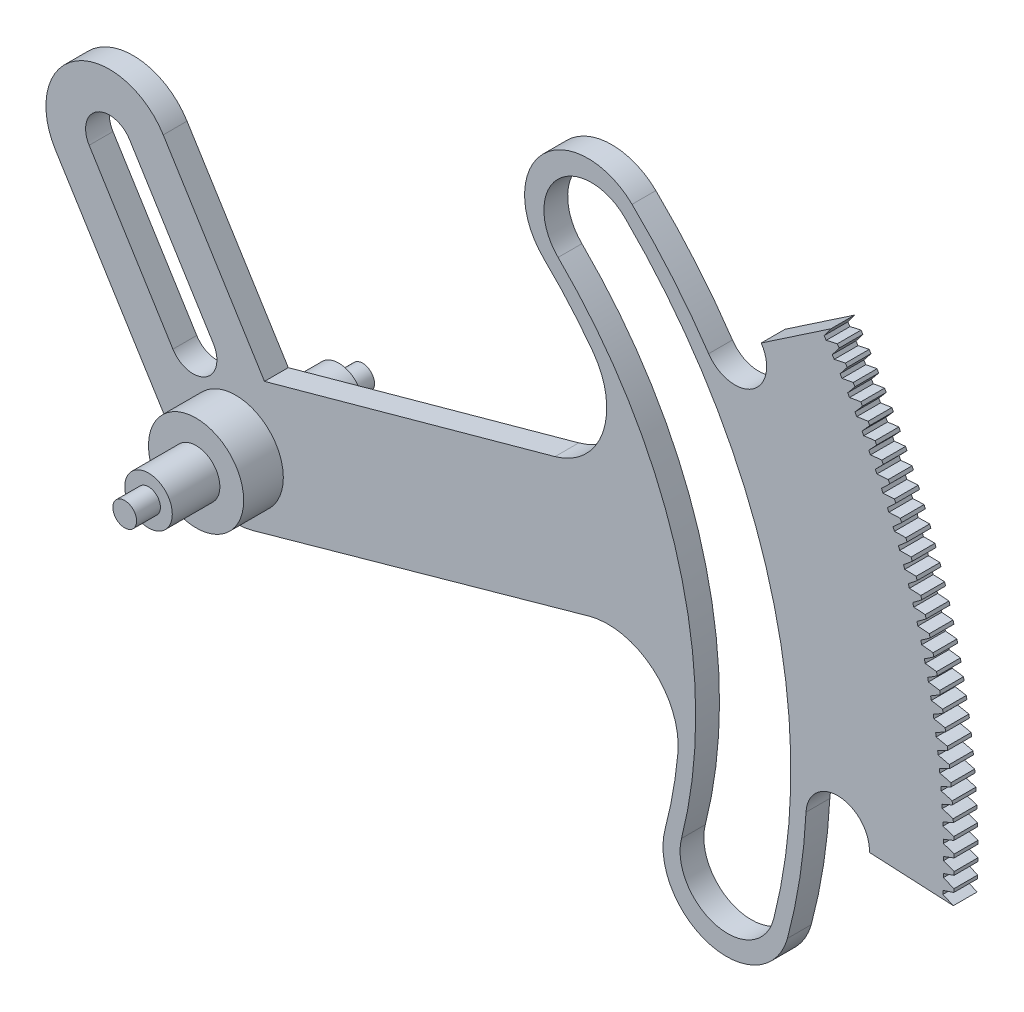
from build123d import *

# Parameters (mm, degrees)
BOSS_EXTRUDE_2_DEPTH = 1.5
BOSS_EXTRUDE_3_DEPTH = 1.5
SKETCH_12_R          = 3
BOSS_EXTRUDE_4_DEPTH = 2.5
SKETCH_13_R          = 1.5
BOSS_EXTRUDE_5_DEPTH = 3
SKETCH_14_R          = 0.75
BOSS_EXTRUDE_6_DEPTH = 1.5
BOSS_EXTRUDE_START   = 5
SKETCH_15_R          = 1.5
BOSS_EXTRUDE_7_DEPTH = 5
BOSS_EXTRUDE_START_2 = 1.5
SKETCH_16_R          = 0.75
BOSS_EXTRUDE_8_DEPTH = 1.5


with BuildPart() as part:
    # Sketch 6 → Boss-Extrude 2 (new body)
    with BuildSketch(Plane.XY):
        with BuildLine():
            Line((37.519779375, 25.38417136), (33.130048014, 22.414279348))
            ThreePointArc((33.130048014, 22.414279348), (32.59425958, 19.63706298), (29.817043212, 20.172851413))
            ThreePointArc((29.817043212, 20.172851413), (34.671419838, 9.689821796), (35.955419193, -1.791041762))
            ThreePointArc((35.955419193, -1.791041762), (38.052444802, 0.106979206), (39.95046577, -1.990046403))
            Line((39.95046577, -1.990046403), (45.243902486, -2.253727551))
            ThreePointArc((45.243902486, -2.253727551), (44.913502165, -2.110667794), (44.580306552, -1.974245108))
            ThreePointArc((44.580306552, -1.974245108), (44.58532509, -1.857461343), (44.590037698, -1.740664833))
            ThreePointArc((44.590037698, -1.740664833), (44.933425979, -1.632429188), (45.274580707, -1.517346967))
            ThreePointArc((45.274580707, -1.517346967), (45.278003129, -1.411535572), (45.281178259, -1.305716468))
            ThreePointArc((45.281178259, -1.305716468), (44.947854383, -1.169607468), (44.611874824, -1.040192624))
            ThreePointArc((44.611874824, -1.040192624), (44.614446527, -0.923329372), (44.6167121, -0.806459783))
            ThreePointArc((44.6167121, -0.806459783), (44.957758354, -0.691056496), (45.29642816, -0.568854908))
            ThreePointArc((45.29642816, -0.568854908), (45.297633885, -0.462995046), (45.298592211, -0.357132655))
            ThreePointArc((45.298592211, -0.357132655), (44.962490986, -0.228034115), (44.623874853, -0.105683879))
            ThreePointArc((44.623874853, -0.105683879), (44.623998593, 0.011207602), (44.623816137, 0.128099005))
            ThreePointArc((44.623816137, 0.128099005), (44.96237077, 0.250619317), (45.298407104, 0.379886669))
            ThreePointArc((45.298407104, 0.379886669), (45.297395602, 0.485748565), (45.296136703, 0.591607808))
            ThreePointArc((45.296136703, 0.591607808), (44.957405555, 0.713639262), (44.616301376, 0.828871224))
            ThreePointArc((44.616301376, 0.828871224), (44.613977098, 0.945739659), (44.611346694, 1.062601605))
            ThreePointArc((44.611346694, 1.062601605), (44.947261204, 1.1921852), (45.280516668, 1.328461615))
            ThreePointArc((45.280516668, 1.328461615), (45.277288384, 1.434279111), (45.273812812, 1.540088773))
            ThreePointArc((45.273812812, 1.540088773), (44.93260032, 1.654999613), (44.589157715, 1.763062756))
            ThreePointArc((44.589157715, 1.763062756), (44.584386438, 1.879856884), (44.579309239, 1.996638113))
            ThreePointArc((44.579309239, 1.996638113), (44.912436284, 2.133228151), (45.242764702, 2.276453854))
            ThreePointArc((45.242764702, 2.276453854), (45.237321051, 2.382180534), (45.231630331, 2.487894204))
            ThreePointArc((45.231630331, 2.487894204), (44.888086161, 2.595634028), (44.542455774, 2.696480953))
            ThreePointArc((44.542455774, 2.696480953), (44.535239593, 2.813149544), (44.527717825, 2.929798833))
            ThreePointArc((44.527717825, 2.929798833), (44.857911284, 3.0733354), (45.185167762, 3.223447568))
            ThreePointArc((45.185167762, 3.223447568), (45.177511134, 3.329037057), (45.169607762, 3.434608365))
            ThreePointArc((45.169607762, 3.434608365), (44.823882604, 3.535129912), (44.476216042, 3.628716381))
            ThreePointArc((44.476216042, 3.628716381), (44.46655812, 3.745208261), (44.456595084, 3.861674442))
            ThreePointArc((44.456595084, 3.861674442), (44.783710122, 4.01209458), (45.107751116, 4.169027369))
            ThreePointArc((45.107751116, 4.169027369), (45.097884867, 4.274433352), (45.08777231, 4.37981599))
            ThreePointArc((45.08777231, 4.37981599), (44.740017811, 4.47307517), (44.39046757, 4.559360135))
            ThreePointArc((44.39046757, 4.559360135), (44.378372145, 4.675624206), (44.36597221, 4.791856194))
            ThreePointArc((44.36597221, 4.791856194), (44.689865345, 4.949093922), (45.010548719, 5.112778496))
            ThreePointArc((45.010548719, 5.112778496), (44.998477178, 5.217954739), (44.986159871, 5.323102483))
            ThreePointArc((44.986159871, 5.323102483), (44.636528568, 5.40905839), (44.285247973, 5.488004003))
            ThreePointArc((44.285247973, 5.488004003), (44.270720349, 5.603989267), (44.255888955, 5.71993608))
            ThreePointArc((44.255888955, 5.71993608), (44.576418116, 5.883922429), (44.893603208, 6.05428699))
            ThreePointArc((44.893603208, 6.05428699), (44.879331669, 6.159187358), (44.864815015, 6.264054088))
            ThreePointArc((44.864815015, 6.264054088), (44.513460267, 6.342669017), (44.160603402, 6.414240651))
            ThreePointArc((44.160603402, 6.414240651), (44.143649953, 6.529896234), (44.126393604, 6.645507012))
            ThreePointArc((44.126393604, 6.645507012), (44.443418197, 6.816170053), (44.756965879, 6.993139873))
            ThreePointArc((44.756965879, 6.993139873), (44.740500602, 7.097718355), (44.723790969, 7.202258071))
            ThreePointArc((44.723790969, 7.202258071), (44.370866892, 7.27349754), (44.016588531, 7.3376638))
            ThreePointArc((44.016588531, 7.3376638), (43.997216692, 7.452938973), (43.977542959, 7.568163005))
            ThreePointArc((43.977542959, 7.568163005), (44.290923926, 7.745427879), (44.600696665, 7.928925334))
            ThreePointArc((44.600696665, 7.928925334), (44.582044873, 8.033136057), (44.56314959, 8.137302906))
            ThreePointArc((44.56314959, 8.137302906), (44.208810988, 8.201135667), (43.85326653, 8.257868408))
            ThreePointArc((43.85326653, 8.257868408), (43.831484798, 8.372712606), (43.80940231, 8.487499352))
            ThreePointArc((43.80940231, 8.487499352), (44.119002192, 8.671288304), (44.424864112, 8.861232906))
            ThreePointArc((44.424864112, 8.861232906), (44.404033986, 8.965030161), (44.382961341, 9.068778451))
            ThreePointArc((44.382961341, 9.068778451), (44.027363639, 9.125176505), (43.670709036, 9.174450842))
            ThreePointArc((43.670709036, 9.174450842), (43.646526966, 9.28881369), (43.622045409, 9.403112801))
            ThreePointArc((43.622045409, 9.403112801), (43.927728405, 9.593345216), (44.229545345, 9.789653649))
            ThreePointArc((44.229545345, 9.789653649), (44.206546021, 9.892991906), (44.183305258, 9.996276131))
            ThreePointArc((44.183305258, 9.996276131), (43.826604433, 10.045214739), (43.468996126, 10.087009059))
            ThreePointArc((43.468996126, 10.087009059), (43.442424325, 10.200840394), (43.415554437, 10.314601734))
            ThreePointArc((43.415554437, 10.314601734), (43.717186465, 10.51119417), (44.014826038, 10.713780326))
            ThreePointArc((44.014826038, 10.713780326), (43.989667605, 10.816614257), (43.964268917, 10.919389113))
            ThreePointArc((43.964268917, 10.919389113), (43.606621429, 10.960846809), (43.248216278, 10.99514278))
            ThreePointArc((43.248216278, 10.99514278), (43.219266401, 11.108392672), (43.190019968, 11.221566342))
            ThreePointArc((43.190019968, 11.221566342), (43.487468721, 11.424432567), (43.780800373, 11.633207585))
            ThreePointArc((43.780800373, 11.633207585), (43.753493867, 11.735492085), (43.725948395, 11.83771249))
            ThreePointArc((43.725948395, 11.83771249), (43.367511121, 11.87167109), (43.008466333, 11.898453668))
            ThreePointArc((43.008466333, 11.898453668), (42.977151078, 12.011072442), (42.945540929, 12.1236088))
            ThreePointArc((42.945540929, 12.1236088), (43.238675937, 12.332659829), (43.527571002, 12.547532134))
            ThreePointArc((43.527571002, 12.547532134), (43.4981284, 12.649222337), (43.468448226, 12.750843455))
            ThreePointArc((43.468448226, 12.750843455), (43.109378388, 12.777288064), (42.749851453, 12.796545501))
            ThreePointArc((42.749851453, 12.796545501), (42.716184556, 12.908483759), (42.682224556, 13.020333443))
            ThreePointArc((42.682224556, 13.020333443), (42.970917241, 13.23547758), (43.255249, 13.456352922))
            ThreePointArc((43.255249, 13.456352922), (43.223683216, 13.557404223), (43.19188136, 13.658381479))
            ThreePointArc((43.19188136, 13.658381479), (42.832336457, 13.677300496), (42.472485075, 13.689024346))
            ThreePointArc((42.472485075, 13.689024346), (42.436481304, 13.800232988), (42.400186349, 13.911346937))
            ThreePointArc((42.400186349, 13.911346937), (42.68431008, 14.132489813), (42.963953816, 14.359271308))
            ThreePointArc((42.963953816, 14.359271308), (42.930278696, 14.459639383), (42.896369107, 14.559928485))
            ThreePointArc((42.896369107, 14.559928485), (42.536506848, 14.571313613), (42.176488862, 14.575498733))
            ThreePointArc((42.176488862, 14.575498733), (42.138164009, 14.685928978), (42.099550019, 14.796258454))
            ThreePointArc((42.099550019, 14.796258454), (42.378980169, 15.023303068), (42.653813222, 15.255891243))
            ThreePointArc((42.653813222, 15.255891243), (42.618043537, 15.355532067), (42.582041088, 15.455089025))
            ThreePointArc((42.582041088, 15.455089025), (42.222019322, 15.45893527), (41.861992646, 15.455579824))
            ThreePointArc((41.861992646, 15.455579824), (41.821363522, 15.565183235), (41.780447434, 15.674679843))
            ThreePointArc((41.780447434, 15.674679843), (42.055061438, 15.907526607), (42.324963256, 16.14581944))
            ThreePointArc((42.324963256, 16.14581944), (42.287114696, 16.244689308), (42.249035179, 16.343470453))
            ThreePointArc((42.249035179, 16.343470453), (41.889011822, 16.339776127), (41.529134377, 16.328881587))
            ThreePointArc((41.529134377, 16.328881587), (41.486218804, 16.437610088), (41.443018565, 16.5462258))
            ThreePointArc((41.443018565, 16.5462258), (41.712695967, 16.784772578), (41.977548162, 17.028665547))
            ThreePointArc((41.977548162, 17.028665547), (41.937637329, 17.126721091), (41.897497447, 17.224683094))
            ThreePointArc((41.897497447, 17.224683094), (41.537630417, 17.213449818), (41.178060058, 17.195020963))
            ThreePointArc((41.178060058, 17.195020963), (41.132876858, 17.302826862), (41.087411418, 17.410514036))
            ThreePointArc((41.087411418, 17.410514036), (41.352033928, 17.654656193), (41.611720328, 17.904042319))
            ThreePointArc((41.611720328, 17.904042319), (41.569764728, 18.001240527), (41.527582088, 18.09834042))
            ThreePointArc((41.527582088, 18.09834042), (41.168029235, 18.07957312), (40.80892368, 18.053618031))
            ThreePointArc((40.80892368, 18.053618031), (40.761492674, 18.160454041), (40.713781975, 18.26716544))
            ThreePointArc((40.713781975, 18.26716544), (40.973233522, 18.51679589), (41.227640219, 18.771565782))
            ThreePointArc((41.227640219, 18.771565782), (41.183658254, 18.867864022), (41.139451359, 18.964059212))
            ThreePointArc((41.139451359, 18.964059212), (40.780370394, 18.937766123), (40.42188716, 18.904296189))
            ThreePointArc((40.42188716, 18.904296189), (40.372229151, 19.010115448), (40.322294121, 19.115804266))
            ThreePointArc((40.322294121, 19.115804266), (40.5764609, 19.370813511), (40.825476304, 19.63085542))
            ThreePointArc((40.825476304, 19.63085542), (40.779487267, 19.726211451), (40.733275507, 19.821459745))
            ThreePointArc((40.733275507, 19.821459745), (40.374823936, 19.787652397), (40.017120264, 19.746682298))
            ThreePointArc((40.017120264, 19.746682298), (39.965257034, 19.85143839), (39.913119577, 19.956058269))
            ThreePointArc((39.913119577, 19.956058269), (40.161890102, 20.216334453), (40.405404986, 20.481534316))
            ThreePointArc((40.405404986, 20.481534316), (40.357429049, 20.575906312), (40.309232694, 20.67016593))
            ThreePointArc((40.309232694, 20.67016593), (39.951567745, 20.628859154), (39.594800536, 20.580406859))
            ThreePointArc((39.594800536, 20.580406859), (39.540754835, 20.684053835), (39.486437819, 20.787558885))
            ThreePointArc((39.486437819, 20.787558885), (39.729702971, 21.052987842), (39.967610521, 21.323229333))
            ThreePointArc((39.967610521, 21.323229333), (39.917668728, 21.4165759), (39.867508919, 21.509805497))
            ThreePointArc((39.867508919, 21.509805497), (39.510787475, 21.461017411), (39.15511322, 21.405104174))
            ThreePointArc((39.15511322, 21.405104174), (39.098908754, 21.507596571), (39.042436004, 21.60994139))
            ThreePointArc((39.042436004, 21.60994139), (39.280089079, 21.880406696), (39.512284942, 22.155571278))
            ThreePointArc((39.512284942, 22.155571278), (39.460399199, 22.24785147), (39.408297938, 22.340010153))
            ThreePointArc((39.408297938, 22.340010153), (39.052676469, 22.283762156), (38.698251178, 22.220412502))
            ThreePointArc((38.698251178, 22.220412502), (38.639912599, 22.321705364), (38.581308886, 22.422845061))
            ThreePointArc((38.581308886, 22.422845061), (38.813245642, 22.698228079), (39.039627968, 22.978195057))
            ThreePointArc((39.039627968, 22.978195057), (38.985821034, 23.069368398), (38.931801174, 23.160415742))
            ThreePointArc((38.931801174, 23.160415742), (38.577435668, 23.096732507), (38.224414803, 23.025974224))
            ThreePointArc((38.224414803, 23.025974224), (38.163967701, 23.126023119), (38.103258731, 23.225913331))
            ThreePointArc((38.103258731, 23.225913331), (38.329377433, 23.50609327), (38.549846924, 23.79073984))
            ThreePointArc((38.549846924, 23.79073984), (38.4941424, 23.880766338), (38.438227635, 23.970662407))
            ThreePointArc((38.438227635, 23.970662407), (38.085273529, 23.899571868), (37.733811937, 23.821435992))
            ThreePointArc((37.733811937, 23.821435992), (37.671282826, 23.920197036), (37.608495228, 24.018793947))
            ThreePointArc((37.608495228, 24.018793947), (37.828696692, 24.303647912), (38.043156642, 24.592849219))
            ThreePointArc((38.043156642, 24.592849219), (37.985578963, 24.681689384), (37.92779382, 24.770394747))
            ThreePointArc((37.92779382, 24.770394747), (37.57640593, 24.691928087), (37.226657774, 24.606448891))
            ThreePointArc((37.226657774, 24.606448891), (37.162074081, 24.703878764), (37.097235396, 24.801139127))
            ThreePointArc((37.097235396, 24.801139127), (37.311423035, 25.09054217), (37.519779375, 25.38417136))
        make_face()
    extrude(amount=BOSS_EXTRUDE_2_DEPTH)

    # Sketch 3 → Boss-Extrude 3 (add)
    with BuildSketch(Plane.XY):
        with BuildLine():
            Line((1.81296518, 4.659956561), (-4.57018681, 14.927549789))
            ThreePointArc((-4.57018681, 14.927549789), (-10.079118229, 16.212724722), (-11.364293163, 10.703793302))
            Line((-11.364293163, 10.703793302), (-3.397053177, -2.111878243))
            ThreePointArc((-3.397053177, -2.111878243), (-1.450313033, -3.727813314), (1.076646897, -3.852379973))
            Line((1.076646897, -3.852379973), (22.264736751, 2.069177957))
            ThreePointArc((22.264736751, 2.069177957), (26.304212974, 1.200877354), (27.877176583, -2.619737724))
            ThreePointArc((27.877176583, -2.619737724), (27.566814633, -4.906193123), (27.069244377, -7.159330197))
            ThreePointArc((27.069244377, -7.159330197), (29.8820925, -12.040922759), (34.786526847, -9.268093113))
            ThreePointArc((34.786526847, -9.268093113), (34.6802111, 9.658310311), (24.988133825, 25.915114662))
            ThreePointArc((24.988133825, 25.915114662), (19.332217326, 25.812116791), (19.435215197, 20.156200293))
            ThreePointArc((19.435215197, 20.156200293), (21.052585969, 18.4604611), (22.522496812, 16.63541816))
            ThreePointArc((22.522496812, 16.63541816), (23.148079682, 12.543236941), (20.129109139, 9.710726055))
            Line((20.129109139, 9.710726055), (1.81296518, 4.659956561))
        make_face()
        with BuildLine():
            Line((-6.693345045, 13.607625887), (-1.413649437, 5.114992944))
            ThreePointArc((-1.413649437, 5.114992944), (-1.895590038, 3.049143662), (-3.96143932, 3.531084262))
            Line((-3.96143932, 3.531084262), (-9.241134928, 12.023717204))
            ThreePointArc((-9.241134928, 12.023717204), (-8.759194328, 14.089566487), (-6.693345045, 13.607625887))
        make_face(mode=Mode.SUBTRACT)
        with BuildLine():
            ThreePointArc((28.104853069, -7.149631738), (27.929754808, 7.80569), (20.325796492, 20.684825282))
            ThreePointArc((20.325796492, 20.684825282), (20.288655583, 24.927303397), (24.531133697, 24.964444306))
            ThreePointArc((24.531133697, 24.964444306), (33.708324768, 9.420660345), (33.919650255, -8.628865891))
            ThreePointArc((33.919650255, -8.628865891), (30.272634585, -10.796647408), (28.104853069, -7.149631738))
        make_face(mode=Mode.SUBTRACT)
    extrude(amount=BOSS_EXTRUDE_3_DEPTH)

    # Sketch 12 → Boss-Extrude 4 (add)
    with BuildSketch(Plane.XY.offset(1.5)):
        Circle(SKETCH_12_R)
    extrude(amount=BOSS_EXTRUDE_4_DEPTH)

    # Sketch 13 → Boss-Extrude 5 (add)
    with BuildSketch(Plane.XY.offset(4)):
        Circle(SKETCH_13_R)
    extrude(amount=BOSS_EXTRUDE_5_DEPTH)

    # Sketch 14 → Boss-Extrude 6 (add)
    with BuildSketch(Plane.XY.offset(7)):
        Circle(SKETCH_14_R)
    extrude(amount=BOSS_EXTRUDE_6_DEPTH)

    # Sketch 15 → Boss-Extrude 7 (add)
    with BuildSketch(Plane(origin=(0, 0, 0), x_dir=(-1, 0, 0), z_dir=(0, 0, -1)).offset(BOSS_EXTRUDE_START)):
        with Locations(Location((0, 0, 0), (0, 0, 180))):
            Circle(SKETCH_15_R)
    extrude(amount=-BOSS_EXTRUDE_7_DEPTH)

    # Sketch 16 → Boss-Extrude 8 (add)
    with BuildSketch(Plane(origin=(0, 0, -5), x_dir=(-1, 0, 0), z_dir=(0, 0, -1)).offset(BOSS_EXTRUDE_START_2)):
        with Locations(Location((0, 0, 0), (0, 0, 180))):
            Circle(SKETCH_16_R)
    extrude(amount=-BOSS_EXTRUDE_8_DEPTH)


solid = part.part
